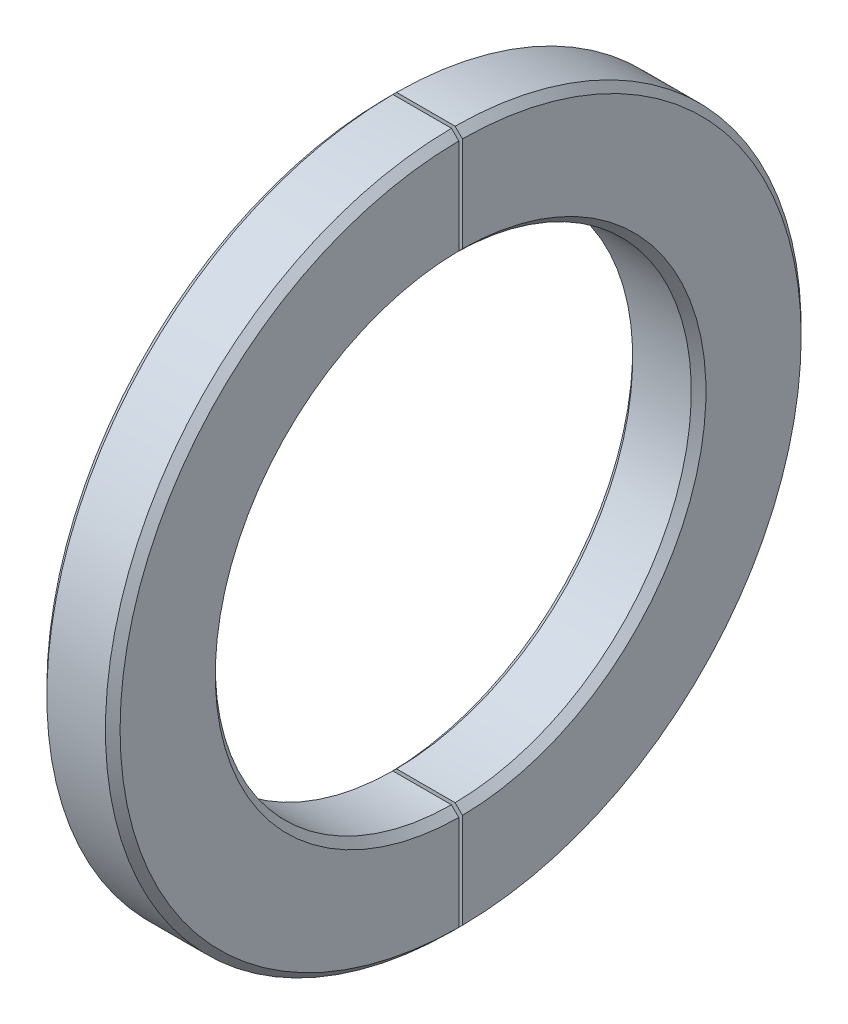
SolidWorks part; units mm, degrees
material "45"
ref_plane "前视基准面" through (0, 0, 0) normal (0, 0, 1) x (1, 0, 0)
ref_plane "上视基准面" through (0, 0, 0) normal (0, 1, 0) x (1, 0, 0)
ref_plane "右视基准面" through (0, 0, 0) normal (1, 0, 0) x (0, 0, -1)
sketch "草图1" plane through (0, 0, 0) normal (1, 0, 0) x (0, 0, -1)
  circle A0 centre (0, 0) radius 32.5
  circle A1 centre (0, 0) radius 47.5
  dimension "D1" = 65
  dimension "D2" = 95
extrude "凸台-拉伸1" add sketch "草图1" along normal blind 10
chamfer "倒角1" distance 1 angle 45 4 edges at (0, 0, -32.5) (10, 0, -32.5) (0, 0, -47.5) (10, 0, -47.5)
sketch "草图2" plane through (0, 0, 0) normal (-1, 0, 0) x (0, 0, 1)
  line L1 (-0.25, 79.6736) -> (0.25, 79.6736)
  line L2 (-0.25, 79.6736) -> (-0.25, -79.6736)
  line L3 (-0.25, -79.6736) -> (0.25, -79.6736)
  line L4 (0.25, 79.6736) -> (0.25, -79.6736)
  line L5 (-0.25, 79.6736) -> (0.25, -79.6736) construction
  line L6 (-0.25, -79.6736) -> (0.25, 79.6736) construction
  point P0 (0, 0)
  dimension "D1" = 0.5
extrude "切除-拉伸1" cut sketch "草图2" against normal through all
equation "\"XMMCDM\"= \"QC名称代码\""
